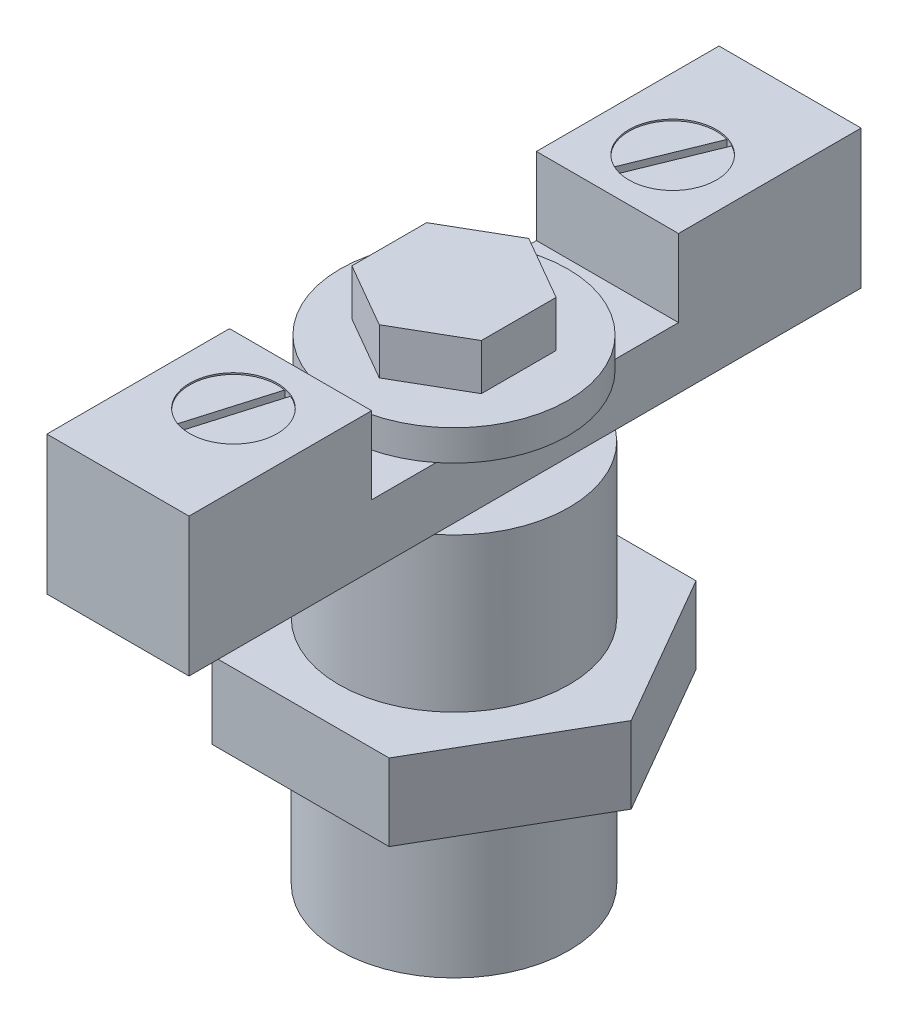
SolidWorks part; units mm, degrees
ref_plane "Front Plane" through (0, 0, 0) normal (0, 0, 1) x (1, 0, 0)
ref_plane "Top Plane" through (0, 0, 0) normal (0, 1, 0) x (1, 0, 0)
ref_plane "Right Plane" through (0, 0, 0) normal (1, 0, 0) x (0, 0, -1)
sketch "Sketch1" plane through (0, 0, 0) normal (0, 1, 0) x (1, 0, 0)
  line L1 (5.7735, 10) -> (-5.7735, 10)
  line L2 (-5.7735, 10) -> (-11.547, 0)
  line L3 (-11.547, 0) -> (-5.7735, -10)
  line L4 (-5.7735, -10) -> (5.7735, -10)
  line L5 (5.7735, -10) -> (11.547, 0)
  line L6 (11.547, 0) -> (5.7735, 10)
  circle A0 centre (0, 0) radius 10 construction
  dimension "D1" = 20
extrude "Boss-Extrude1" add sketch "Sketch1" along normal blind 5
sketch "Sketch2" plane through (0, 0, 0) normal (0, -1, 0) x (1, 0, 0)
  circle A0 centre (0, 0) radius 7.5
  dimension "D1" = 15
extrude "Boss-Extrude2" add sketch "Sketch2" along normal blind 10
sketch "Sketch9" plane through (0, 5, 0) normal (0, 1, 0) x (1, 0, 0)
  circle A1 centre (0, 0) radius 7.5
  circle A2 centre (0, 0) radius 7.5
  dimension "D1" = 0
extrude "Boss-Extrude7" add sketch "Sketch9" along normal blind 10
sketch "Sketch3" plane through (0, 15, 0) normal (0, 1, 0) x (1, 0, 0)
  line L1 (-4.6309, -21.9) -> (4.6309, -21.9)
  line L2 (-4.6309, -21.9) -> (-4.6309, 21.9)
  line L3 (-4.6309, 21.9) -> (4.6309, 21.9)
  line L4 (4.6309, -21.9) -> (4.6309, 21.9)
  line L5 (-4.6309, -21.9) -> (4.6309, 21.9) construction
  line L6 (-4.6309, 21.9) -> (4.6309, -21.9) construction
  point P0 (0, 0)
  dimension "D1" = 43.8
extrude "Boss-Extrude3" add sketch "Sketch3" along normal blind 4
sketch "Sketch4" plane through (0, 19, 0) normal (0, 1, 0) x (1, 0, 0)
  line L1 (-4.6309, 21.9) -> (4.6309, 21.9)
  line L2 (-4.6309, 21.9) -> (-4.6309, 10)
  line L3 (-4.6309, 10) -> (4.6309, 10)
  line L4 (4.6309, 21.9) -> (4.6309, 10)
  line L5 (-4.6309, -21.9) -> (4.6309, -21.9)
  line L6 (-4.6309, -21.9) -> (-4.6309, -10)
  line L7 (-4.6309, -10) -> (4.6309, -10)
  line L8 (4.6309, -21.9) -> (4.6309, -10)
extrude "Boss-Extrude4" add sketch "Sketch4" along normal blind 5.03
sketch "Sketch5" plane through (0, 19, 0) normal (0, 1, 0) x (1, 0, 0)
  circle A0 centre (0, 0) radius 7.424
extrude "Boss-Extrude5" add sketch "Sketch5" along normal blind 2
sketch "Sketch6" plane through (0, 21, 0) normal (0, 1, 0) x (1, 0, 0)
  line L1 (0, 4.8711) -> (-4.2185, 2.4355)
  line L2 (-4.2185, 2.4355) -> (-4.2185, -2.4355)
  line L3 (-4.2185, -2.4355) -> (0, -4.8711)
  line L4 (0, -4.8711) -> (4.2185, -2.4355)
  line L5 (4.2185, -2.4355) -> (4.2185, 2.4355)
  line L6 (4.2185, 2.4355) -> (0, 4.8711)
  circle A0 centre (0, 0) radius 4.2185 construction
extrude "Boss-Extrude6" add sketch "Sketch6" along normal blind 3
sketch "Sketch7" plane through (0, 24.03, 0) normal (0, 1, 0) x (1, 0, 0)
  circle A0 centre (0, 14.2505) radius 2.8507
  circle A1 centre (0, -14.3728) radius 2.8507
extrude "Cut-Extrude1" cut sketch "Sketch7" against normal blind 0.1
sketch "Sketch8" plane through (0, 23.93, 0) normal (0, 1, 0) x (1, 0, 0)
  line L0 (-1.3431, 11.7193) -> (0.8043, 17.0008)
  line L1 (-1.3431, 11.7193) -> (-0.8167, 11.5053)
  line L2 (0.8043, 17.0008) -> (1.3307, 16.7868)
  line L3 (-0.8167, 11.5053) -> (1.3307, 16.7868)
  line L4 (-1.3431, 11.7193) -> (1.3307, 16.7868) construction
  line L5 (0.8043, 17.0008) -> (-0.8167, 11.5053) construction
  line L6 (-1.0769, -17.0275) -> (0.5318, -11.5578)
  line L7 (-1.0769, -17.0275) -> (-0.5318, -17.1878)
  line L8 (0.5318, -11.5578) -> (1.0769, -11.7181)
  line L9 (-0.5318, -17.1878) -> (1.0769, -11.7181)
  line L10 (-1.0769, -17.0275) -> (1.0769, -11.7181) construction
  line L11 (0.5318, -11.5578) -> (-0.5318, -17.1878) construction
  point P1 (-0.0062, 14.253)
  point P2 (0, -14.3728)
extrude "Cut-Extrude2" cut sketch "Sketch8" against normal blind 1
